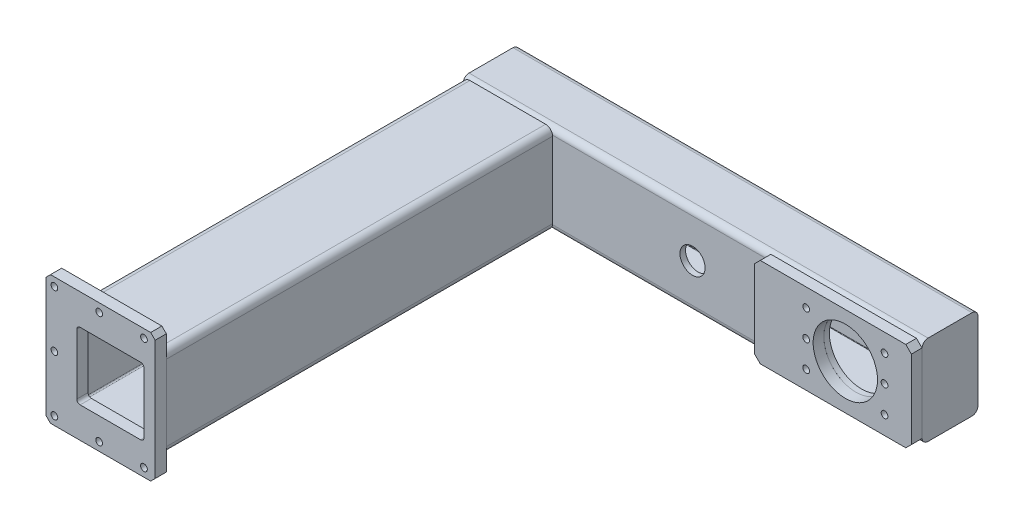
from build123d import *

# Parameters (mm, degrees)
STRUCTURAL_MEMBER1_DEPTH            = 740
STRUCTURAL_MEMBER2_DEPTH            = 740
BODY_START                          = 370
BODY_2_RUN_ON_DEPTH                 = 450
SKETCH6_W                           = 195
SKETCH6_H                           = 230
BOSS_EXTRUDE3_DEPTH                 = 20
SKETCH7_W                           = 280
SKETCH7_H                           = 160
BOSS_EXTRUDE4_DEPTH                 = 19
SKETCH12_R                          = 57.5
CUT_EXTRUDE1_DEPTH                  = 88
SKETCH13_R                          = 6
CUT_EXTRUDE2_DEPTH                  = 30
SKETCH14_R                          = 41
SKETCH14_R_2                        = 22.5
CUT_EXTRUDE3_DEPTH                  = 1104.143236393
CIRPATTERN1_COUNT                   = 4
LPATTERN1_COUNT                     = 2
LPATTERN1_PITCH                     = 622
SKETCH17_W                          = 43
SKETCH17_H                          = 100
SKETCH17_W_2                        = 225
SKETCH17_W_3                        = 192
CUT_EXTRUDE4_DEPTH                  = 10
FILLET1_R                           = 6
CIRPATTERN2_COUNT                   = 4
SKETCH21_W                          = 115
SKETCH21_H                          = 115
CUT_EXTRUDE6_DEPTH                  = 51
FILLET2_R                           = 6
SKETCH22_W                          = 82.362058938
SKETCH22_H                          = 143.177077148
BOSS_EXTRUDE9_DEPTH                 = 5
SKETCH23_W                          = 81.720401824
SKETCH23_H                          = 143.403473864
BOSS_EXTRUDE10_DEPTH                = 5
M4_TAPPED_HOLE2_AT_2_COUNT          = 2
M4_TAPPED_HOLE2_AT_2_PITCH          = 90
M4_TAPPED_HOLE2_AT_3_COUNT          = 2
M4_TAPPED_HOLE2_AT_3_PITCH          = 289.352725925
M4_TAPPED_HOLE2_AT_4_COUNT          = 2
M4_TAPPED_HOLE2_AT_4_PITCH          = 275
M4_TAPPED_HOLE2_AT_5_COUNT          = 2
M4_TAPPED_HOLE2_AT_5_PITCH          = 512
M4_TAPPED_HOLE2_AT_6_COUNT          = 2
M4_TAPPED_HOLE2_AT_6_PITCH          = 519.849978359
M4_TAPPED_HOLE2_AT_7_COUNT          = 2
M4_TAPPED_HOLE2_AT_7_PITCH          = 628.477525453
M4_TAPPED_HOLE2_AT_8_COUNT          = 2
M4_TAPPED_HOLE2_AT_8_PITCH          = 622
M4_TAPPED_HOLE2_AT_9_COUNT          = 2
M4_TAPPED_HOLE2_AT_9_PITCH          = 675.296231294
M4_TAPPED_HOLE2_AT_10_COUNT         = 2
M4_TAPPED_HOLE2_AT_10_PITCH         = 678.619923079
SKETCH26_W                          = 6
SKETCH26_H                          = 810
F_12_0_12_DIAMETER_HOLE1_AT_2_COUNT = 2
F_12_0_12_DIAMETER_HOLE1_AT_2_PITCH = 80
F_12_0_12_DIAMETER_HOLE1_AT_3_COUNT = 2
F_12_0_12_DIAMETER_HOLE1_AT_3_PITCH = 160
F_12_0_12_DIAMETER_HOLE1_AT_4_COUNT = 2
F_12_0_12_DIAMETER_HOLE1_AT_4_PITCH = 200
F_12_0_12_DIAMETER_HOLE1_AT_5_COUNT = 2
F_12_0_12_DIAMETER_HOLE1_AT_5_PITCH = 215.406592285
F_12_0_12_DIAMETER_HOLE1_AT_6_COUNT = 2
F_12_0_12_DIAMETER_HOLE1_AT_6_PITCH = 256.124969497
F_12_0_12_DIAMETER_HOLE1_AT_7_COUNT = 2
F_12_0_12_DIAMETER_HOLE1_AT_7_PITCH = 100
CHAMFER1_SIZE                       = 8
CHAMFER2_SIZE                       = 10
SKETCH28_W                          = 120
SKETCH28_H                          = 120
CUT_EXTRUDE7_DEPTH                  = 65
FILLET3_R                           = 6


with BuildPart() as part:
    # Sketch1 → Structural Member1 (new body)
    with BuildSketch(Plane.XY):
        with BuildLine():
            Line((-67.607270131, -80), (67.607270131, -80))
            ThreePointArc((67.607270131, -80), (76.370253459, -76.370253459), (80, -67.607270131))
            Line((80, -67.607270131), (80, 67.607270131))
            ThreePointArc((80, 67.607270131), (76.370253459, 76.370253459), (67.607270131, 80))
            Line((67.607270131, 80), (-67.607270131, 80))
            ThreePointArc((-67.607270131, 80), (-76.370253459, 76.370253459), (-80, 67.607270131))
            Line((-80, 67.607270131), (-80, -67.607270131))
            ThreePointArc((-80, -67.607270131), (-76.370253459, -76.370253459), (-67.607270131, -80))
        make_face()
        with BuildLine():
            Line((-67.607270131, -70), (67.607270131, -70))
            ThreePointArc((67.607270131, -70), (69.299185647, -69.299185647), (70, -67.607270131))
            Line((70, -67.607270131), (70, 67.607270131))
            ThreePointArc((70, 67.607270131), (69.299185647, 69.299185647), (67.607270131, 70))
            Line((67.607270131, 70), (-67.607270131, 70))
            ThreePointArc((-67.607270131, 70), (-69.299185647, 69.299185647), (-70, 67.607270131))
            Line((-70, 67.607270131), (-70, -67.607270131))
            ThreePointArc((-70, -67.607270131), (-69.299185647, -69.299185647), (-67.607270131, -70))
        make_face(mode=Mode.SUBTRACT)
    extrude(amount=STRUCTURAL_MEMBER1_DEPTH)

    # Trim/Extend1
    split(bisect_by=Plane(origin=(370, 0, 50), x_dir=(0, -1, 0), z_dir=(0, 0, 1)), keep=Keep.TOP)


with BuildPart() as body_2:
    # Sketch11 → Structural Member2 (new body)
    with BuildSketch(Plane(origin=(0, 0, 0), x_dir=(0, 0, -1), z_dir=(1, 0, 0))):
        with BuildLine():
            Line((-39.214127736, -80), (39.214127736, -80))
            ThreePointArc((39.214127736, -80), (46.840891155, -76.840891155), (50, -69.214127736))
            Line((50, -69.214127736), (50, 69.214127736))
            ThreePointArc((50, 69.214127736), (46.840891155, 76.840891155), (39.214127736, 80))
            Line((39.214127736, 80), (-39.214127736, 80))
            ThreePointArc((-39.214127736, 80), (-46.840891155, 76.840891155), (-50, 69.214127736))
            Line((-50, 69.214127736), (-50, -69.214127736))
            ThreePointArc((-50, -69.214127736), (-46.840891155, -76.840891155), (-39.214127736, -80))
        make_face()
        with BuildLine():
            Line((-39.214127736, -70), (39.214127736, -70))
            ThreePointArc((39.214127736, -70), (39.769823343, -69.769823343), (40, -69.214127736))
            Line((40, -69.214127736), (40, 69.214127736))
            ThreePointArc((40, 69.214127736), (39.769823343, 69.769823343), (39.214127736, 70))
            Line((39.214127736, 70), (-39.214127736, 70))
            ThreePointArc((-39.214127736, 70), (-39.769823343, 69.769823343), (-40, 69.214127736))
            Line((-40, 69.214127736), (-40, -69.214127736))
            ThreePointArc((-40, -69.214127736), (-39.769823343, -69.769823343), (-39.214127736, -70))
        make_face(mode=Mode.SUBTRACT)
    extrude(amount=STRUCTURAL_MEMBER2_DEPTH)

    # body 2 cut square before the run-on
    split(bisect_by=Plane.YZ.offset(370), keep=Keep.TOP)

    # Sketch11 → body 2 run on (add)
    with BuildSketch(Plane(origin=(0, 0, 0), x_dir=(0, 0, -1), z_dir=(1, 0, 0)).offset(BODY_START)):
        with BuildLine():
            Line((-39.214127736, -80), (39.214127736, -80))
            ThreePointArc((39.214127736, -80), (46.840891155, -76.840891155), (50, -69.214127736))
            Line((50, -69.214127736), (50, 69.214127736))
            ThreePointArc((50, 69.214127736), (46.840891155, 76.840891155), (39.214127736, 80))
            Line((39.214127736, 80), (-39.214127736, 80))
            ThreePointArc((-39.214127736, 80), (-46.840891155, 76.840891155), (-50, 69.214127736))
            Line((-50, 69.214127736), (-50, -69.214127736))
            ThreePointArc((-50, -69.214127736), (-46.840891155, -76.840891155), (-39.214127736, -80))
        make_face()
        with BuildLine():
            Line((-39.214127736, -70), (39.214127736, -70))
            ThreePointArc((39.214127736, -70), (39.769823343, -69.769823343), (40, -69.214127736))
            Line((40, -69.214127736), (40, 69.214127736))
            ThreePointArc((40, 69.214127736), (39.769823343, 69.769823343), (39.214127736, 70))
            Line((39.214127736, 70), (-39.214127736, 70))
            ThreePointArc((-39.214127736, 70), (-39.769823343, 69.769823343), (-40, 69.214127736))
            Line((-40, 69.214127736), (-40, -69.214127736))
            ThreePointArc((-40, -69.214127736), (-39.769823343, -69.769823343), (-39.214127736, -70))
        make_face(mode=Mode.SUBTRACT)
    extrude(amount=-BODY_2_RUN_ON_DEPTH)


with BuildPart() as body_3:
    # Sketch6 → Boss-Extrude3 (new body)
    with BuildSketch(Plane.XY.offset(740)):
        with Locations((-17.5, 0)):
            Rectangle(SKETCH6_W, SKETCH6_H)
    extrude(amount=BOSS_EXTRUDE3_DEPTH)

    # Sketch26 → Ø12.0 (12) Diameter Hole1 (revolve, cut)
    with BuildSketch(Plane(origin=(-100, -100, 760), x_dir=(0, -1, 0), z_dir=(1, 0, 0))):
        with Locations((3, 405)):
            Rectangle(SKETCH26_W, SKETCH26_H)
    f_12_0_12_diameter_hole1 = revolve(axis=Axis((-100, -100, 766.35), (0, 0, -1)), mode=Mode.SUBTRACT)

    # Ø12.0 (12) Diameter Hole1 at 2: Ø12.0 (12) Diameter Hole1 ×2
    with Locations(*[(i * F_12_0_12_DIAMETER_HOLE1_AT_2_PITCH, 0, 0) for i in range(1, F_12_0_12_DIAMETER_HOLE1_AT_2_COUNT)]):
        add(f_12_0_12_diameter_hole1, mode=Mode.SUBTRACT)

    # Ø12.0 (12) Diameter Hole1 at 3: Ø12.0 (12) Diameter Hole1 ×2
    with Locations(*[(i * F_12_0_12_DIAMETER_HOLE1_AT_3_PITCH, 0, 0) for i in range(1, F_12_0_12_DIAMETER_HOLE1_AT_3_COUNT)]):
        add(f_12_0_12_diameter_hole1, mode=Mode.SUBTRACT)

    # Ø12.0 (12) Diameter Hole1 at 4: Ø12.0 (12) Diameter Hole1 ×2
    with Locations(*[(0, i * F_12_0_12_DIAMETER_HOLE1_AT_4_PITCH, 0) for i in range(1, F_12_0_12_DIAMETER_HOLE1_AT_4_COUNT)]):
        add(f_12_0_12_diameter_hole1, mode=Mode.SUBTRACT)

    # Ø12.0 (12) Diameter Hole1 at 5: Ø12.0 (12) Diameter Hole1 ×2
    with Locations(*[Vector(0.3713906763541037, 0.9284766908852593, 0) * (i * F_12_0_12_DIAMETER_HOLE1_AT_5_PITCH) for i in range(1, F_12_0_12_DIAMETER_HOLE1_AT_5_COUNT)]):
        add(f_12_0_12_diameter_hole1, mode=Mode.SUBTRACT)

    # Ø12.0 (12) Diameter Hole1 at 6: Ø12.0 (12) Diameter Hole1 ×2
    with Locations(*[Vector(0.6246950475544243, 0.7808688094430304, 0) * (i * F_12_0_12_DIAMETER_HOLE1_AT_6_PITCH) for i in range(1, F_12_0_12_DIAMETER_HOLE1_AT_6_COUNT)]):
        add(f_12_0_12_diameter_hole1, mode=Mode.SUBTRACT)

    # Ø12.0 (12) Diameter Hole1 at 7: Ø12.0 (12) Diameter Hole1 ×2
    with Locations(*[(0, i * F_12_0_12_DIAMETER_HOLE1_AT_7_PITCH, 0) for i in range(1, F_12_0_12_DIAMETER_HOLE1_AT_7_COUNT)]):
        add(f_12_0_12_diameter_hole1, mode=Mode.SUBTRACT)

    # Chamfer1
    chamfer1_edges = [body_3.edges().sort_by_distance(p)[0] for p in [
        (-115, 115, 750),
        (80, 115, 750),
        (80, -115, 750),
        (-115, -115, 750),
    ]]
    chamfer(chamfer1_edges, length=CHAMFER1_SIZE)

    # Sketch28 → Cut-Extrude7 (cut)
    with BuildSketch(Plane.XY.offset(760)):
        Rectangle(SKETCH28_W, SKETCH28_H)
    extrude(amount=-CUT_EXTRUDE7_DEPTH, mode=Mode.SUBTRACT)

    # Fillet3
    fillet3_edges = [body_3.edges().sort_by_distance(p)[0] for p in [
        (-60, -60, 750),
        (-60, 60, 750),
        (60, 60, 750),
        (60, -60, 750),
    ]]
    fillet(fillet3_edges, radius=FILLET3_R)


with BuildPart() as body_4:
    # Sketch7 → Boss-Extrude4 (new body)
    with BuildSketch(Plane.XY.offset(50)):
        with Locations((600, 0)):
            Rectangle(SKETCH7_W, SKETCH7_H)
    extrude(amount=BOSS_EXTRUDE4_DEPTH)


with BuildPart() as cut_extrude1_tool:
    # Sketch12 → Cut-Extrude1 (new body)
    with BuildSketch(Plane.XY.offset(69)):
        with Locations((622, 0)):
            Circle(SKETCH12_R)
    extrude(amount=-CUT_EXTRUDE1_DEPTH)


with BuildPart() as body_2_1:
    add(body_2.part)

    # Cut-Extrude1: cut by cut_extrude1_tool
    add(cut_extrude1_tool.part, mode=Mode.SUBTRACT)


with BuildPart() as body_4_1:
    add(body_4.part)

    # Cut-Extrude1: cut by cut_extrude1_tool
    add(cut_extrude1_tool.part, mode=Mode.SUBTRACT)


with BuildPart() as cut_extrude2_tool:
    # Sketch13 → Cut-Extrude2 (new body)
    with BuildSketch(Plane.XY.offset(69)):
        with Locations((692, 47.5)):
            Circle(SKETCH13_R)
        with Locations((692, 0)):
            Circle(SKETCH13_R)
        with Locations((692, -47.5)):
            Circle(SKETCH13_R)
        with Locations((552, 47.5)):
            Circle(SKETCH13_R)
        with Locations((552, 0)):
            Circle(SKETCH13_R)
        with Locations((552, -47.5)):
            Circle(SKETCH13_R)
    extrude(amount=-CUT_EXTRUDE2_DEPTH)


with BuildPart() as body_2_2:
    add(body_2_1.part)

    # Cut-Extrude2: cut by cut_extrude2_tool
    add(cut_extrude2_tool.part, mode=Mode.SUBTRACT)

    # Sketch14 → Cut-Extrude3 (cut, through all)
    with BuildSketch(Plane(origin=(0, 0, -50), x_dir=(-1, 0, 0), z_dir=(0, 0, -1))):
        with Locations((-622, 0)):
            Circle(SKETCH14_R)
        with Locations((-330, 0)):
            Circle(SKETCH14_R_2)
        Circle(SKETCH14_R)
    extrude(amount=-CUT_EXTRUDE3_DEPTH, mode=Mode.SUBTRACT)

    # Sketch15 → M6 Tapped Hole1 (revolve, cut)
    with BuildSketch(Plane(origin=(622, -52.5, -50), x_dir=(0, 1, 0), z_dir=(1, 0, 0))):
        Polygon((0, 0), (0, 16.502151548), (2.5, 15), (2.5, 0), align=None)
    m6_tapped_hole1 = revolve(axis=Axis((622, -52.5, -56.35), (0, 0, 1)), mode=Mode.SUBTRACT)

    # CirPattern1: M6 Tapped Hole1 ×4 about axis
    cirpattern1_axis = Axis((622, 0, 0), (0, 0, 1))
    for i in range(1, CIRPATTERN1_COUNT):
        add(m6_tapped_hole1.rotate(cirpattern1_axis, i * 360 / CIRPATTERN1_COUNT), mode=Mode.SUBTRACT)

    # LPattern1: M6 Tapped Hole1 ×2
    with Locations(*[(-i * LPATTERN1_PITCH, 0, 0) for i in range(1, LPATTERN1_COUNT)]):
        add(m6_tapped_hole1, mode=Mode.SUBTRACT)

    # LPattern1 copy 1 sketch → LPattern1 copy 1 (revolve, cut)
    with BuildSketch(Plane(origin=(52.5, 0, -50), x_dir=(-1, 0, 0), z_dir=(0, 1, 0))):
        Polygon((0, 0), (0, 16.502151548), (2.5, 15), (2.5, 0), align=None)
    revolve(axis=Axis((52.5, 0, -56.35), (0, 0, 1)), mode=Mode.SUBTRACT)

    # LPattern1 copy 2 sketch → LPattern1 copy 2 (revolve, cut)
    with BuildSketch(Plane(origin=(0, 52.5, -50), x_dir=(0, -1, 0), z_dir=(-1, 0, 0))):
        Polygon((0, 0), (0, 16.502151548), (2.5, 15), (2.5, 0), align=None)
    revolve(axis=Axis((0, 52.5, -56.35), (0, 0, 1)), mode=Mode.SUBTRACT)

    # LPattern1 copy 3 sketch → LPattern1 copy 3 (revolve, cut)
    with BuildSketch(Plane(origin=(-52.5, 0, -50), x_dir=(1, 0, 0), z_dir=(0, -1, 0))):
        Polygon((0, 0), (0, 16.502151548), (2.5, 15), (2.5, 0), align=None)
    revolve(axis=Axis((-52.5, 0, -56.35), (0, 0, 1)), mode=Mode.SUBTRACT)

    # Sketch17 → Cut-Extrude4 (cut)
    with BuildSketch(Plane(origin=(0, 0, -50), x_dir=(-1, 0, 0), z_dir=(0, 0, -1))):
        with Locations((-703.5, 0)):
            Rectangle(SKETCH17_W, SKETCH17_H)
        with Locations((-177.5, 0)):
            Rectangle(SKETCH17_W_2, SKETCH17_H)
        with Locations((-466, 0)):
            Rectangle(SKETCH17_W_3, SKETCH17_H)
    extrude(amount=-CUT_EXTRUDE4_DEPTH, mode=Mode.SUBTRACT)

    # Fillet1
    fillet1_edges = [body_2_2.edges().sort_by_distance(p)[0] for p in [
        (725, -50, -45),
        (725, 50, -45),
        (682, 50, -45),
        (682, -50, -45),
        (290, -50, -45),
        (290, 50, -45),
        (65, 50, -45),
        (65, -50, -45),
        (370, 50, -45),
        (370, -50, -45),
        (562, -50, -45),
        (562, 50, -45),
    ]]
    fillet(fillet1_edges, radius=FILLET1_R)

    # Sketch18 → M4 Tapped Hole1 (revolve, cut)
    with BuildSketch(Plane(origin=(355.5, -25.5, -50), x_dir=(0, 1, 0), z_dir=(1, 0, 0))):
        Polygon((0, 0), (0, 11.091420021), (1.65, 10.1), (1.65, 0), align=None)
    m4_tapped_hole1 = revolve(axis=Axis((355.5, -25.5, -56.35), (0, 0, 1)), mode=Mode.SUBTRACT)

    # CirPattern2: M4 Tapped Hole1 ×4 about axis
    cirpattern2_axis = Axis((330, 0, 0), (0, 0, 1))
    for i in range(1, CIRPATTERN2_COUNT):
        add(m4_tapped_hole1.rotate(cirpattern2_axis, i * 360 / CIRPATTERN2_COUNT), mode=Mode.SUBTRACT)

    # Sketch21 → Cut-Extrude6 (cut)
    with BuildSketch(Plane(origin=(0, 0, 40), x_dir=(-1, 0, 0), z_dir=(0, 0, -1))):
        Rectangle(SKETCH21_W, SKETCH21_H)
    extrude(amount=-CUT_EXTRUDE6_DEPTH, mode=Mode.SUBTRACT)

    # Fillet2
    fillet2_edges = [body_2_2.edges().sort_by_distance(p)[0] for p in [
        (-57.5, 57.5, 45),
        (-57.5, -57.5, 45),
        (57.5, -57.5, 45),
        (57.5, 57.5, 45),
    ]]
    fillet(fillet2_edges, radius=FILLET2_R)

    # Sketch22 → Boss-Extrude9 (add)
    with BuildSketch(Plane.ZY.offset(80)):
        Rectangle(SKETCH22_W, SKETCH22_H)
    extrude(amount=-BOSS_EXTRUDE9_DEPTH)

    # Sketch23 → Boss-Extrude10 (add)
    with BuildSketch(Plane(origin=(740, 0, 0), x_dir=(0, 0, -1), z_dir=(1, 0, 0))):
        Rectangle(SKETCH23_W, SKETCH23_H)
    extrude(amount=-BOSS_EXTRUDE10_DEPTH)

    # Sketch24 → M4 Tapped Hole2 (revolve, cut)
    with BuildSketch(Plane(origin=(55, -45, -50), x_dir=(0, 1, 0), z_dir=(1, 0, 0))):
        Polygon((0, 0), (0, 11.091420021), (1.65, 10.1), (1.65, 0), align=None)
    m4_tapped_hole2 = revolve(axis=Axis((55, -45, -56.35), (0, 0, 1)), mode=Mode.SUBTRACT)

    # M4 Tapped Hole2 at 2: M4 Tapped Hole2 ×2
    with Locations(*[(0, i * M4_TAPPED_HOLE2_AT_2_PITCH, 0) for i in range(1, M4_TAPPED_HOLE2_AT_2_COUNT)]):
        add(m4_tapped_hole2, mode=Mode.SUBTRACT)

    # M4 Tapped Hole2 at 3: M4 Tapped Hole2 ×2
    with Locations(*[Vector(0.9503971290446889, 0.31103906041462553, 0) * (i * M4_TAPPED_HOLE2_AT_3_PITCH) for i in range(1, M4_TAPPED_HOLE2_AT_3_COUNT)]):
        add(m4_tapped_hole2, mode=Mode.SUBTRACT)

    # M4 Tapped Hole2 at 4: M4 Tapped Hole2 ×2
    with Locations(*[(i * M4_TAPPED_HOLE2_AT_4_PITCH, 0, 0) for i in range(1, M4_TAPPED_HOLE2_AT_4_COUNT)]):
        add(m4_tapped_hole2, mode=Mode.SUBTRACT)

    # M4 Tapped Hole2 at 5: M4 Tapped Hole2 ×2
    with Locations(*[(i * M4_TAPPED_HOLE2_AT_5_PITCH, 0, 0) for i in range(1, M4_TAPPED_HOLE2_AT_5_COUNT)]):
        add(m4_tapped_hole2, mode=Mode.SUBTRACT)

    # M4 Tapped Hole2 at 6: M4 Tapped Hole2 ×2
    with Locations(*[Vector(0.9848995312379942, 0.1731268707254288, 0) * (i * M4_TAPPED_HOLE2_AT_6_PITCH) for i in range(1, M4_TAPPED_HOLE2_AT_6_COUNT)]):
        add(m4_tapped_hole2, mode=Mode.SUBTRACT)

    # M4 Tapped Hole2 at 7: M4 Tapped Hole2 ×2
    with Locations(*[Vector(0.989693306138984, 0.1432032114992099, 0) * (i * M4_TAPPED_HOLE2_AT_7_PITCH) for i in range(1, M4_TAPPED_HOLE2_AT_7_COUNT)]):
        add(m4_tapped_hole2, mode=Mode.SUBTRACT)

    # M4 Tapped Hole2 at 8: M4 Tapped Hole2 ×2
    with Locations(*[(i * M4_TAPPED_HOLE2_AT_8_PITCH, 0, 0) for i in range(1, M4_TAPPED_HOLE2_AT_8_COUNT)]):
        add(m4_tapped_hole2, mode=Mode.SUBTRACT)

    # M4 Tapped Hole2 at 9: M4 Tapped Hole2 ×2
    with Locations(*[Vector(0.9995613313382166, 0.02961663203965082, 0) * (i * M4_TAPPED_HOLE2_AT_9_PITCH) for i in range(1, M4_TAPPED_HOLE2_AT_9_COUNT)]):
        add(m4_tapped_hole2, mode=Mode.SUBTRACT)

    # M4 Tapped Hole2 at 10: M4 Tapped Hole2 ×2
    with Locations(*[Vector(0.9946657577296573, 0.10315052302381626, 0) * (i * M4_TAPPED_HOLE2_AT_10_PITCH) for i in range(1, M4_TAPPED_HOLE2_AT_10_COUNT)]):
        add(m4_tapped_hole2, mode=Mode.SUBTRACT)


with BuildPart() as body_4_2:
    add(body_4_1.part)

    # Cut-Extrude2: cut by cut_extrude2_tool
    add(cut_extrude2_tool.part, mode=Mode.SUBTRACT)

    # Chamfer2
    chamfer2_edges = [body_4_2.edges().sort_by_distance(p)[0] for p in [
        (460, 80, 59.5),
        (740, 80, 59.5),
        (740, -80, 59.5),
        (460, -80, 59.5),
    ]]
    chamfer(chamfer2_edges, length=CHAMFER2_SIZE)


solid = Compound([part.part, body_3.part, body_2_2.part, body_4_2.part])
